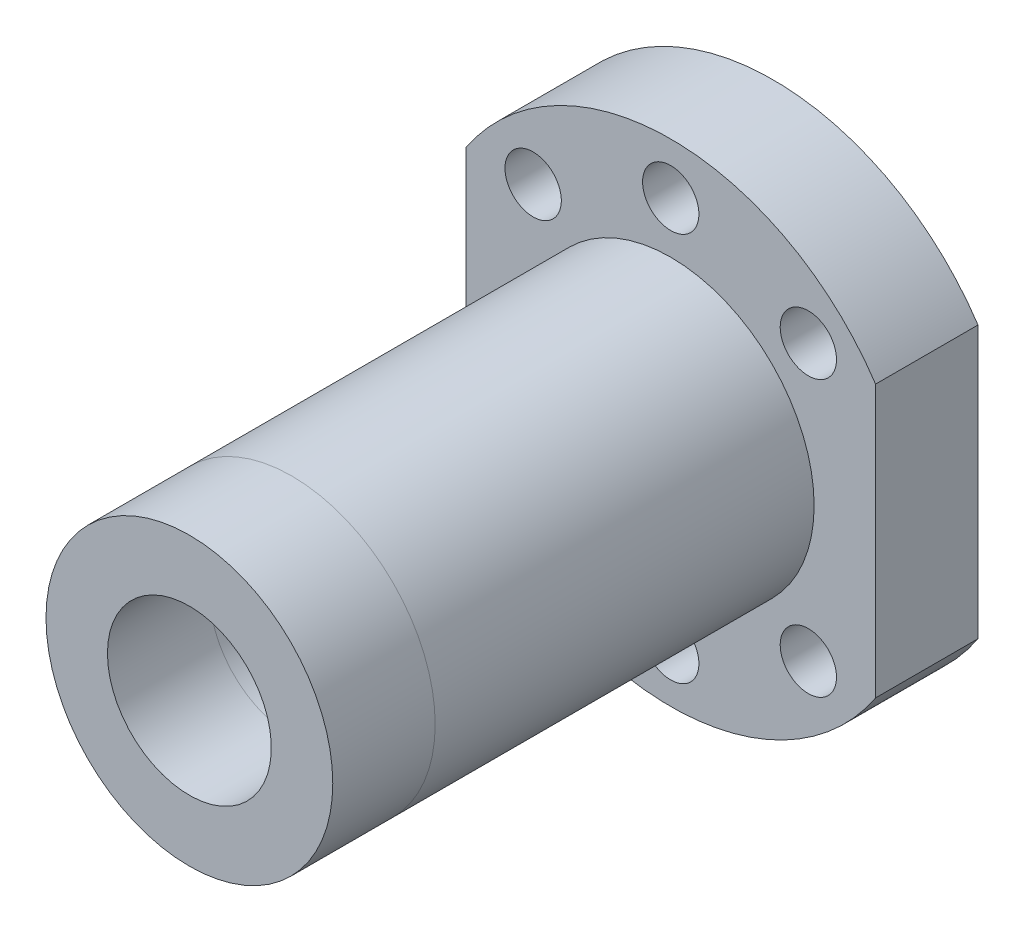
SolidWorks part; units mm, degrees
ref_plane "Front Plane" through (0, 0, 0) normal (0, 0, 1) x (1, 0, 0)
ref_plane "Top Plane" through (0, 0, 0) normal (0, 1, 0) x (1, 0, 0)
ref_plane "Right Plane" through (0, 0, 0) normal (1, 0, 0) x (0, 0, -1)
sketch "Sketch1" plane through (0, 0, 0) normal (0, 0, 1) x (1, 0, 0)
  circle A0 centre (0, 0) radius 14
  circle A1 centre (0, 0) radius 8
  dimension "D1" = 28
  dimension "D2" = 16
extrude "Boss-Extrude1" add sketch "Sketch1" along normal blind 57
sketch "Sketch2" plane through (0, 0, 0) normal (0, 0, -1) x (-1, 0, 0)
  line L1 (-20, 35.3595) -> (20, 35.3595)
  line L2 (-20, 35.3595) -> (-20, -47.1461)
  line L3 (-20, -47.1461) -> (20, -47.1461)
  line L4 (20, 35.3595) -> (20, -47.1461)
  circle A0 centre (0, 0) radius 24
  circle A1 centre (0, 0) radius 8
  circle M1 centre (0, 0) radius 14
  circle M2 centre (0, 0) radius 8
  dimension "D1" = 48
  dimension "D2" = 20
  dimension "D3" = 20
extrude "Boss-Extrude2" add sketch "Sketch2" against normal blind 10 contours L4 A0 L2 M1 | M1 M2
hole_wizard "Ø5.5 (5.5) Diameter Hole1" positions "Sketch4" profile "Sketch5" hole size "Ø5.5" standard "GB" end condition through all
sketch "Sketch4" plane through (0, 0, 0) normal (0, 0, -1) x (-1, 0, 0)
  line L0 (0, 19) -> (0, 0) construction
  line L1 (0, 0) -> (13.435, 13.435) construction
  line L4 (-13.435, 13.435) -> (0, 0) construction
  point P1 (0, 19)
  point P3 (-13.435, 13.435)
  point P5 (13.435, 13.435)
  dimension "D1" = 19
  dimension "D2" = 19
  dimension "D3" = 19
  dimension "D4" = 45
  dimension "D5" = 45
sketch "Sketch5" plane through (0, 19, 0) normal (1, 0, 0) x (0, 1, 0)
  line L0 (0, 0) -> (0, 57)
  line L1 (0, 57) -> (2.75, 57)
  line L2 (2.75, 57) -> (2.75, 0)
  line L5 (2.75, 0) -> (0, 0)
  line L11 (0, -6.35) -> (0, 107.95) construction
  dimension "通孔孔直径" = 5.5
  dimension "通孔孔深度" = 57
mirror "Mirror1" about plane through (0, 0, 0) normal (0, 1, 0) of "Ø5.5 (5.5) Diameter Hole1"
sketch "Sketch6" plane through (0, 0, 0) normal (0, 1, 0) x (1, 0, 0)
  line L0 (-14, -57) -> (14, -57) construction
  line L1 (-26.1493, -10) -> (31.0442, -10)
  line L2 (-26.1493, -10) -> (-26.1493, -47)
  line L3 (-26.1493, -47) -> (31.0442, -47)
  line L4 (31.0442, -10) -> (31.0442, -47)
  line L5 (-20, -10) -> (20, -10) construction
  dimension "D1" = 10
  dimension "D2" = 0
split "Split1" trim tools "Sketch6" resulting bodies 105 106 107
